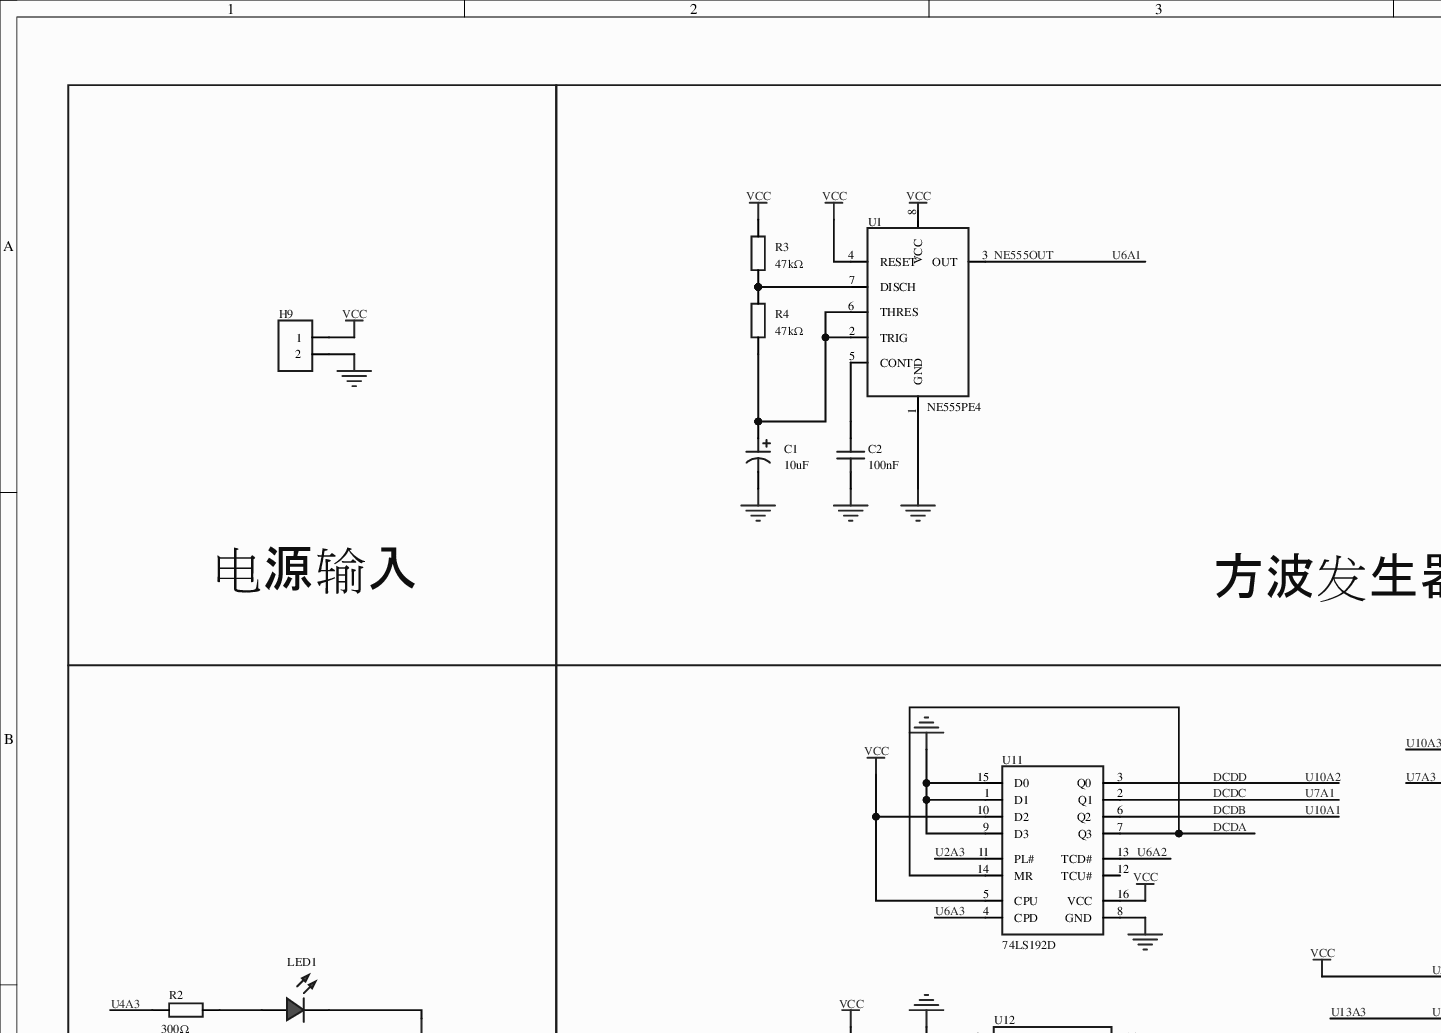
[diagram p0: MISC51493-3.schdoc, top left]
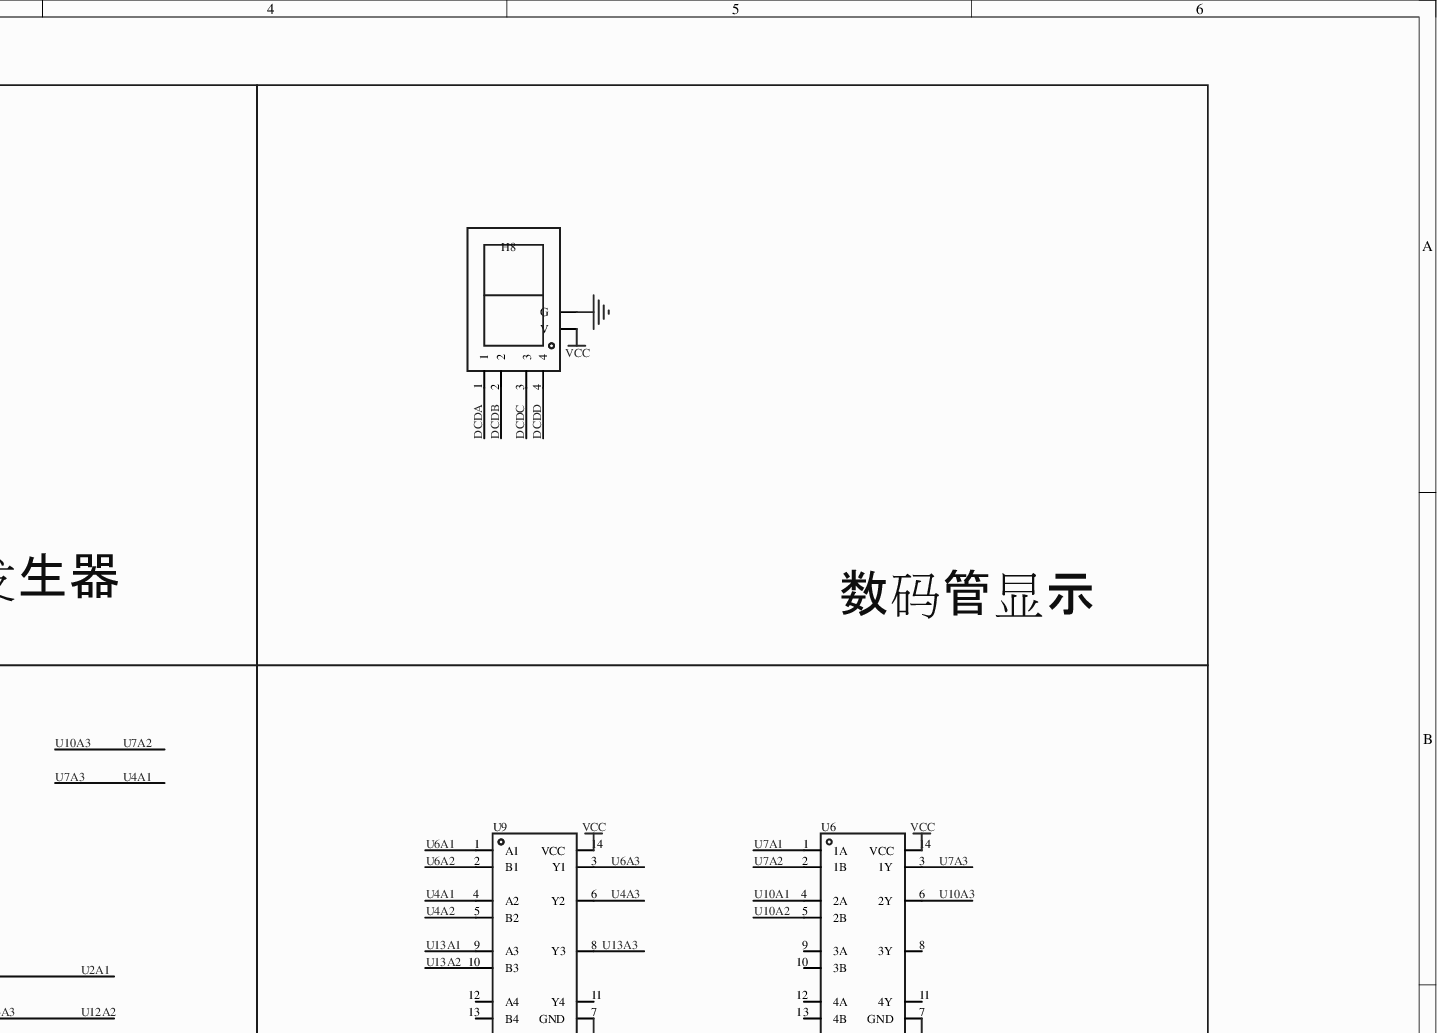
[diagram p1: MISC51493-3.schdoc, top right]
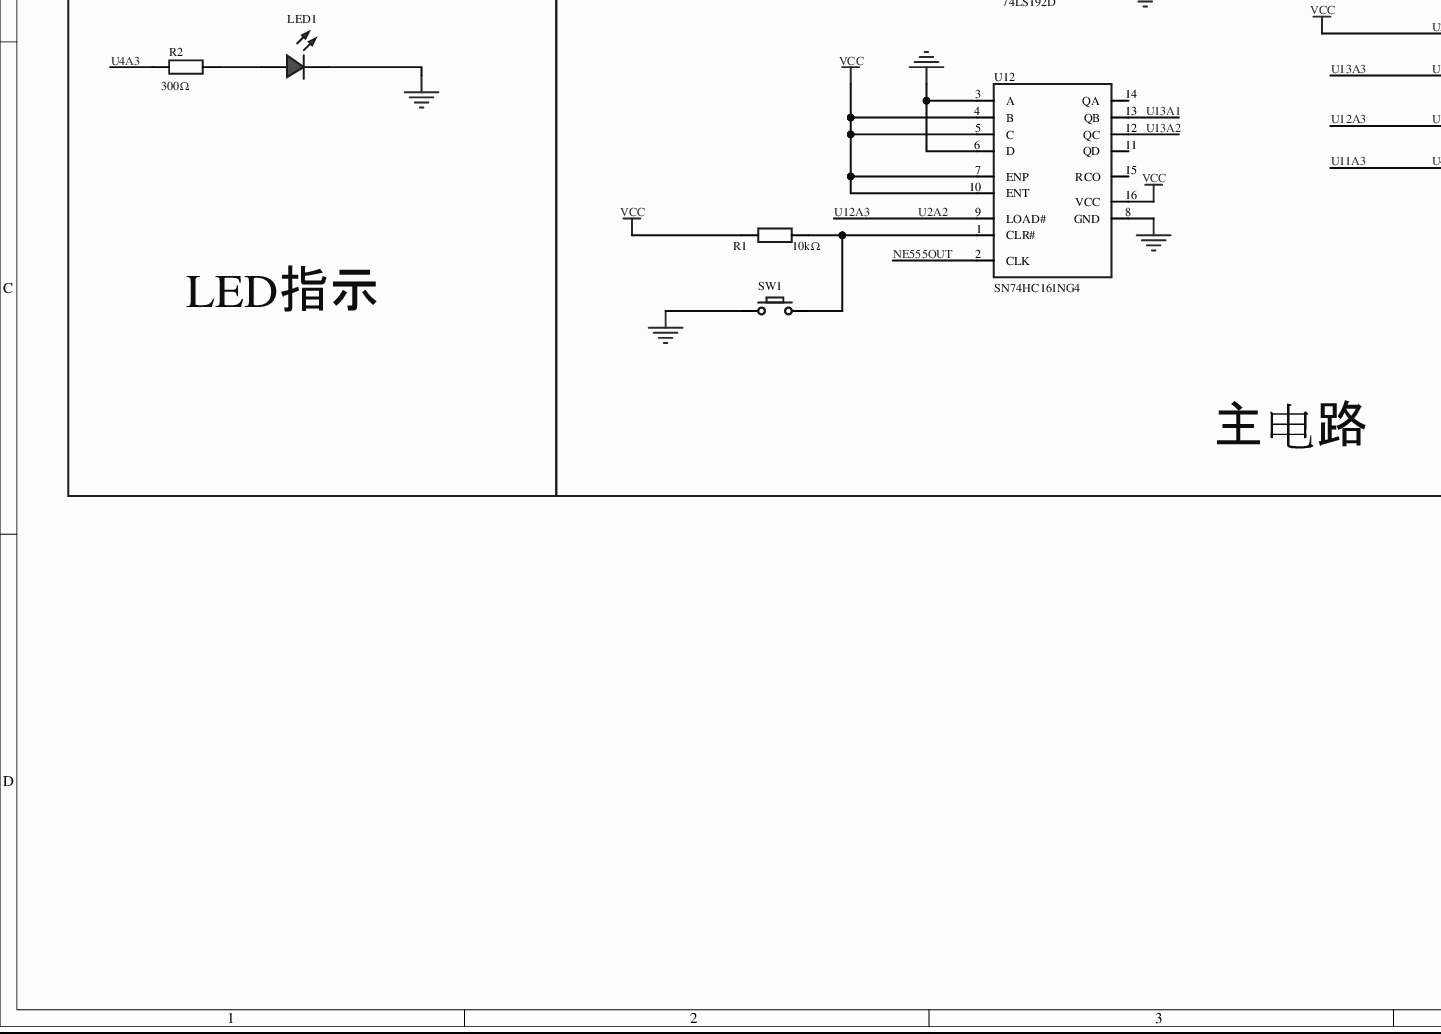
[diagram p2: MISC51493-3.schdoc, bottom left]
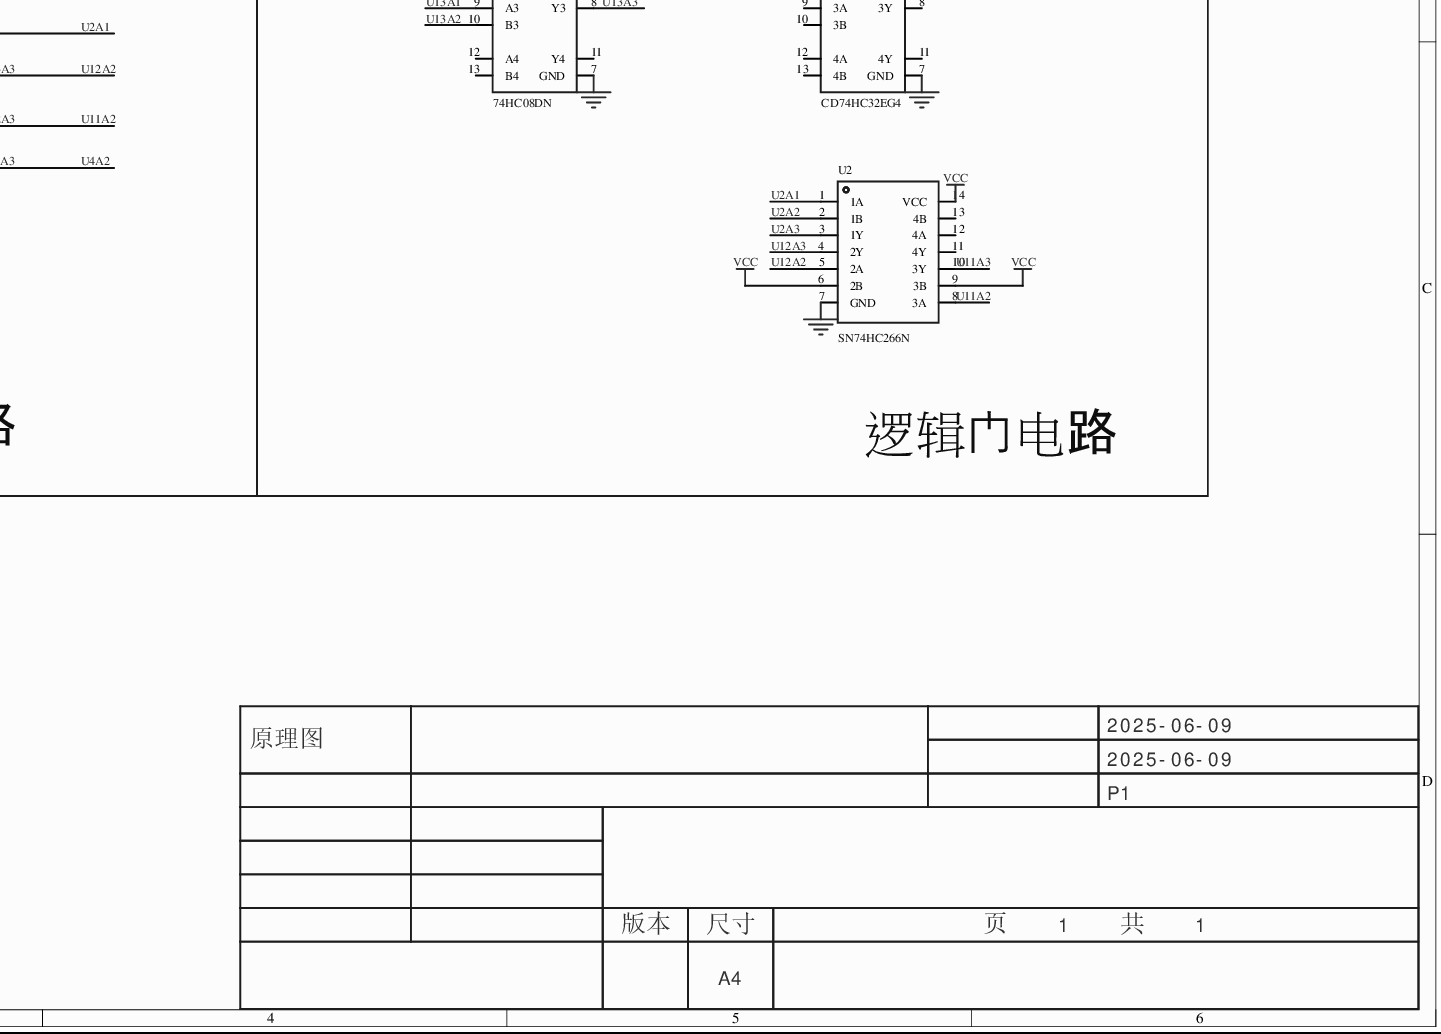
[diagram p3: MISC51493-3.schdoc, bottom right]
# Altium project MISC51493-2.PrjPcb
1 sheet, 16 parts. Net scope: global (net labels, ports and power ports of the same name join across sheets).
Board file: MISC51493.pcbdoc

## Sheet MISC51493-3.schdoc
size 420 x 297 mm; Version: V1.0; @Project Name: MISC51493; @Page Count: 1; @Update Date: 2025-06-09; @Create Date: 2025-06-09; @Schematic Name: MISC51493; @Page No: 1; @Create Time: 11:54:45; @Update Time: 19:54:45; @Board Name: MISC51493

### Parts
C1  10uF  [CAP-TH_BD5.0-P2.00-D0.5-FD]
C2  100nF  [CAP-TH_L4.5-W3.0-P2.50-D0.5]
H8  (no value)  [HDR-TH_6P-P2.54-V-M-1]
H9  (no value)  [HDR-TH_2P-P2.54-V-F]
LED1  (no value)  [LED_TH-3mm]
R1  10kΩ  [Res_1/8W]
R2  300Ω  [Res_1/8W]
R3  47kΩ  [Res_1/8W]
R4  47kΩ  [Res_1/8W]
SW1  (no value)  [Key_TH_3.5x6x4.3]
U1  NE555PE4  [PDIP-8_L9.6-W6.4-P2.54-LS7.9-BL-1]
U2  SN74HC266N  [PDIP-14_L19.3-W6.4-P2.54-LS7.6-BL]
U6  CD74HC32EG4  [PDIP-14_L19.3-W6.4-P2.54-LS7.6-BL]
U9  74HC08DN  [PDIP-14_L19.3-W6.5-P2.54-LS7.6-BL]
U11  74LS192D  [PDIP-16_L19.3-W6.4-P2.54-LS7.94-BL]
U12  SN74HC161NG4  [PDIP-16_L19.3-W6.4-P2.54-LS7.9-BL]

### Nets
GND: C1.2 C2.1 H8.6(G) H9.2 LED1.2(A) SW1.A U1.1(GND) U2.7(GND) U6.7(GND) U9.7(GND) U11.1(D1) U11.8(GND) U11.9(D3) U11.15(D0) U12.3(A) U12.6(D) U12.8(GND)
VCC: H8.5(V) H9.1 R1.1 R3.2 U1.4(RESET) U1.8(VCC) U2.1(1A) U2.6(2B) U2.9(3B) U2.14(VCC) U6.14(VCC) U9.14(VCC) U11.5(CPU) U11.10(D2) U11.16(VCC) U12.4(B) U12.5(C) U12.7(ENP) U12.10(ENT) U12.16(VCC)  [also labelled U2A1]
DCDA: H8.1 U11.7(Q3) U11.14(MR)
DCDB: H8.2 U6.4(2A) U11.6(Q2)  [also labelled U10A1]
DCDC: H8.3 U6.1(1A) U11.2(Q1)  [also labelled U7A1]
DCDD: H8.4 U6.5(2B) U11.3(Q0)  [also labelled U10A2]
NE555OUT: U1.3(OUT) U9.1(A1) U12.2(CLK)  [also labelled U6A1]
U2A3: U2.3(1Y) U11.11(PL#)
U4A1: U6.3(1Y) U9.4(A2)  [also labelled U7A3]
U4A3: R2.2 U9.6(Y2)
U6A2: U9.2(B1) U11.13(TCD#)
U6A3: U9.3(Y1) U11.4(CPD)
U10A3: U6.2(1B) U6.6(2Y)  [also labelled U7A2]
U11A2: U2.2(1B) U2.4(2Y) U2.8(3A) U12.9(LOAD#)  [also labelled U12A3, U2A2]
U11A3: U2.10(3Y) U9.5(B2)  [also labelled U4A2]
U12A2: U2.5(2A) U9.8(Y3)  [also labelled U13A3]
U13A1: U9.9(A3) U12.13(QB)
U13A2: U9.10(B3) U12.12(QC)
NetC1_1: C1.1 R4.1 U1.2(TRIG) U1.6(THRES)
NetC2_2: C2.2 U1.5(CONT)
NetLED1_1: LED1.1(C) R2.1
NetR1_2: R1.2 SW1.B U12.1(CLR#)
NetR3_1: R3.1 R4.2 U1.7(DISCH)

Not connected (* = marked no-connect by the designer): U2 11(4Y)* 12(4A)* 13(4B)*; U6 8(3Y)* 9(3A)* 10(3B)* 11(4Y)* 12(4A)* 13(4B)*; U9 11(Y4)* 12(A4)* 13(B4)*; U11 12(TCU#)*; U12 11(QD)* 14(QA)* 15(RCO)*

### Notes on the sheet
- 电源输入
- 方波发生器
- 数码管显示
- LED指示
- 主电路
- 逻辑门电路
- 2025-06-09
- 原理图
- P1
- 版本
- 尺寸
- A4
- 页    1    共    1

### Library data of the parts
C1 = SHG63V10UF03EC0822: 容值:10uF;精度:±20%;额定电压:63V;; AddInBom: yes; ModelId: aba3b94bdab6406eb4f45c9c765c730e; ModelTransform: 196.85,196.517,0,0,0,0,0,0,-196.85; Tolerance: ±20%; Voltage Rating: 63V; Symbol: SHG63V10UF03EC0822; Device: SHG63V10UF03EC0822; LCSC Part Name: 停产 10uF ±20% 63V; SupplierPart: C5263880; ManufacturerPart: SHG63V10UF03EC0822; Supplier Footprint: 插件,D5xL11mm; JLCPCB Part Class: 扩展库; Datasheet: https://atta.szlcsc.com/upload/public/pdf/source/20221206/74D9A2C5191757C58A566DD8357A6A8B.pdf; Supplier: LCSC; ConvertToPcb: yes; FootprintName: CAP-TH_BD5.0-P2.00-D0.5-FD; ModelName: CAP-TH_BD5.0-P2.00-D0.5-FD; Value: 10uF; Diameter: 5mm; Height - Seated (Max): 11mm
C2 = FA14X8R1H104KNU00: 容值:100nF;精度:±10%;额定电压:50V;温度系数:X8R;; Manufacturer: TDK; AddInBom: yes; ModelId: 4f3b11b509834e358e085933e775514f; ModelTransform: 217.61949,118.11,0,0,0,0,0,0,-196.85; Tolerance: ±10%; Voltage Rated: 50V; Temperature Coefficient: X8R; Symbol: FA14X8R1H104KNU00; Device: FA14X8R1H104KNU00; LCSC Part Name: 100nF ±10% 50V; SupplierPart: C1629759; ManufacturerPart: FA14X8R1H104KNU00; Supplier Footprint: 插件; JLCPCB Part Class: 扩展库; Datasheet: https://atta.szlcsc.com/upload/public/pdf/source/20210503/3ED621F3684B6FF62914AEB5593A787B.pdf; Supplier: LCSC; ConvertToPcb: yes; FootprintName: CAP-TH_L4.5-W3.0-P2.50-D0.5; ModelName: CAP-TH_L4.5-W3.0-P2.50-D0.5; Value: 100nF
H8 = HDR-M_2.54_1x6P: Symbol: Header-Male-2.54_1x6; ConvertToPcb: yes; ModelId: 60739dffc9b04830a286435b0fefbd4a; ModelName: HDR2.54-M-LI-1X6P; ModelTransform: 599.999,100,0,0,0,0,0,0,-118.11; Device: HDR-M_2.54_1x6P; AddInBom: yes; SupplierPart: C37208; Supplier Footprint: 插件; FootprintName: HDR-TH_6P-P2.54-V-M-1
H9 = HDR-F_2.54_1x2P: Symbol: Header-Female-2.54_1x2; ConvertToPcb: yes; ModelId: a9450ef445564560a104363b9aacde4e; ModelName: HDR-TH_2P-P2.54-F-LI-1X2P; ModelTransform: 215.7476,98.425,0,0,0,0,0,0,-129.921; Device: HDR-F_2.54_1x2P; AddInBom: yes; SupplierPart: C49661; Supplier Footprint: 插件; FootprintName: HDR-TH_2P-P2.54-V-F
LED1 = LED_TH-R_3mm: ConvertToPcb: yes; ModelId: a497c992633541038a38947cdc58012f; ModelName: LED-TH-3mm_R; ModelTransform: 141.274,153.327,0,0,0,0,-5.984,0,-137.795; Symbol: LED_TH-R; Device: LED_TH-R_3mm; AddInBom: yes; FootprintName: LED_TH-3mm; Supplier Footprint: 插件
R1-R4 = Res_AXIAL-1/8W: ConvertToPcb: yes; SymbolName: 电阻; ModelId: b2b5ae7ae4c642178fe0039925c86a3f; ModelName: RES-TH_BD1.8-L3.2-P7.20-D0.4; ModelTransform: 282.86,66.88,253.09,0,0,0,0,0,-191; Device: Res_AXIAL-1/8W; AddInBom: yes; Supplier Footprint: 轴向引线; FootprintName: Res_1/8W
  R1: Value: 10kΩ
  R2: Value: 300Ω
  R3 R4: Value: 47kΩ
SW1 = Key_TH_3.5x6x4.3: ConvertToPcb: yes; ModelId: c3523f9014d949d7ba5445190a3178990819f05c4eef4c71ace90d822a990e87; ModelName: SW-TH_L6.0-W3.5-H5.0-P6.5; ModelTransform: 308.49,137.8,335.08,0,0,0,0,0,-129.92; Device: Key_TH_3.5x6x4.3; AddInBom: yes; Supplier Footprint: 插件; SymbolName: Key_TH_3.5x6x4.3; FootprintName: Key_TH_3.5x6x4.3
U1 = NE555PE4: 单精度计时器 8-PDIP 0 to 70; Manufacturer: TI(德州仪器); AddInBom: yes; ModelId: 1b8eaf096e7944deafe216467068c10e; ModelTransform: 377.952,318.897,0,0,0,0,0,0,-118.11; Symbol: NE555PE4; Device: NE555PE4; LCSC Part Name: NE555PE4; SupplierPart: C2859604; ManufacturerPart: NE555PE4; Supplier Footprint: PDIP-8; Datasheet: https://www.ti.com/cn/lit/gpn/sa555; Supplier: LCSC; ConvertToPcb: yes; FootprintName: PDIP-8_L9.6-W6.4-P2.54-LS7.9-BL-1; ModelName: PDIP-8_L9.6-W6.4-P2.54-LS7.9-BL-1
U2 = SN74HC266N: 逻辑类型:异或非门;通道数:4;电源电压:2V~6V;静态电流(最大值):2uA;最大传播延迟:23ns@6V,50pF;; Manufacturer: TI(德州仪器); AddInBom: yes; ModelId: ca4ed987146b49a5a2d3ca847d6466c4; ModelTransform: 755.904,309.842,0,0,0,0,0,0,-125.984; Logic Gate Type: 异或非门; Number of Channels: 4; Supply Voltage: 2V~6V; Quiescent Current (Max): 2uA; Sink Current: 5.2mA; High Level Range (VIH): 1.5V~4.2V; Low Level Range (VIL): 500mV~1.8V; Symbol: SN74HC266N; Device: SN74HC266N; LCSC Part Name: SN74HC266N; SupplierPart: C2867246; ManufacturerPart: SN74HC266N; Supplier Footprint: PDIP-14; JLCPCB Part Class: 扩展库; Datasheet: https://www.ti.com/cn/lit/gpn/sn74hc266; Supplier: LCSC; ConvertToPcb: yes; FootprintName: PDIP-14_L19.3-W6.4-P2.54-LS7.6-BL; ModelName: PDIP-14_L19.3-W6.4-P2.54-LS7.6-BL; Series: 74HC系列; Propagation Delay Time: 23ns@6V,50pF; Operating Temperature: -40℃~+85℃
U6 = CD74HC32EG4: AddInBom: yes; ModelId: ca4ed987146b49a5a2d3ca847d6466c4; ModelTransform: 755.904,309.842,0,0,0,0,0,0,-125.984; Symbol: CD74HC32EG4; Device: CD74HC32EG4; LCSC Part Name: CD74HC32EG4; SupplierPart: C21785722; ManufacturerPart: CD74HC32EG4; Supplier Footprint: -; Supplier: LCSC; ConvertToPcb: yes; FootprintName: PDIP-14_L19.3-W6.4-P2.54-LS7.6-BL; ModelName: PDIP-14_L19.3-W6.4-P2.54-LS7.6-BL
U9 = 74HC08DN: 逻辑类型:与门;; Manufacturer: HGSEMI(华冠); AddInBom: yes; ModelId: 7604059b31ae49f98a0332a7cce2343e; ModelTransform: 759.15391,311.417,0,0,0,0,0,0,-129.921; Logic Gate Type: 与门; Symbol: 74HC08DN; Device: 74HC08DN; LCSC Part Name: 74HC08DN; SupplierPart: C19193443; ManufacturerPart: 74HC08DN; Supplier Footprint: DIP-14; JLCPCB Part Class: 扩展库; Datasheet: https://atta.szlcsc.com/upload/public/pdf/source/20231208/7E987F15538D0197C204C64CB1F7EFCE.pdf; Supplier: LCSC; ConvertToPcb: yes; FootprintName: PDIP-14_L19.3-W6.5-P2.54-LS7.6-BL; ModelName: PDIP-14_L19.3-W6.5-P2.54-LS7.6-BL
U11 = SN74LS192N(LX): 工作电压:2V~6V;元件数:1;触发沿:上升沿;计数速率:24MHz;; Manufacturer: LX(灵星芯微); AddInBom: yes; Logic Type: 10分频; Direction: 向下计数器；向上计数器; Voltage - Supply: 2V~6V; Number of Elements: 1; Trigger Type: 上升沿; Reset: 异步; Timing: 同步; Count Rate: 24MHz; ModelId: 96ff5d01b3074dd183bcbc4cd00a63de; ModelTransform: 759.841,322.44,0,0,0,0,0,0,-137.795; Manufacturer Part: 74LS192D; Symbol: SN74LS192N(LX); Device: SN74LS192N(LX); LCSC Part Name: SN74LS192N(LX); SupplierPart: C22449628; Supplier Footprint: DIP-16; JLCPCB Part Class: 扩展库; Datasheet: https://atta.szlcsc.com/upload/public/pdf/source/20240603/08E986A67799FBEA7E290B817BAE27A9.pdf; Supplier: LCSC; ConvertToPcb: yes; Operating Temperature: -40℃~+85℃; FootprintName: PDIP-16_L19.3-W6.4-P2.54-LS7.94-BL; ModelName: PDIP-16_L19.3-W6.4-P2.54-LS7.94-BL
U12 = SN74HC161NG4: 工作电压:2V~6V;元件数:1;触发沿:上升沿;计数速率:36MHz;; Manufacturer: TI(德州仪器); AddInBom: yes; Logic Type: 二进制计数器; Direction: 向上计数器; Supply Voltage: 2V~6V; Number of Elements: 1; Trigger Type: 上升沿; Reset Style: 异步; Timing mode: 同步; Count Rate: 36MHz; ModelId: 7f4af0d2434d4264b3d074b3c8a801b5; ModelTransform: 759.841,311.023,0,0,0,0,0,-0.001,-129.921; Symbol: SN74HC161NG4; Device: SN74HC161NG4; LCSC Part Name: 36MHz 4位二进制计数器; SupplierPart: C1548034; ManufacturerPart: SN74HC161NG4; Supplier Footprint: PDIP-16; JLCPCB Part Class: 扩展库; Supplier: LCSC; ConvertToPcb: yes; Operating Temperature: -40℃~+85℃; FootprintName: PDIP-16_L19.3-W6.4-P2.54-LS7.9-BL; ModelName: PDIP-16_L19.3-W6.4-P2.54-LS7.9-BL